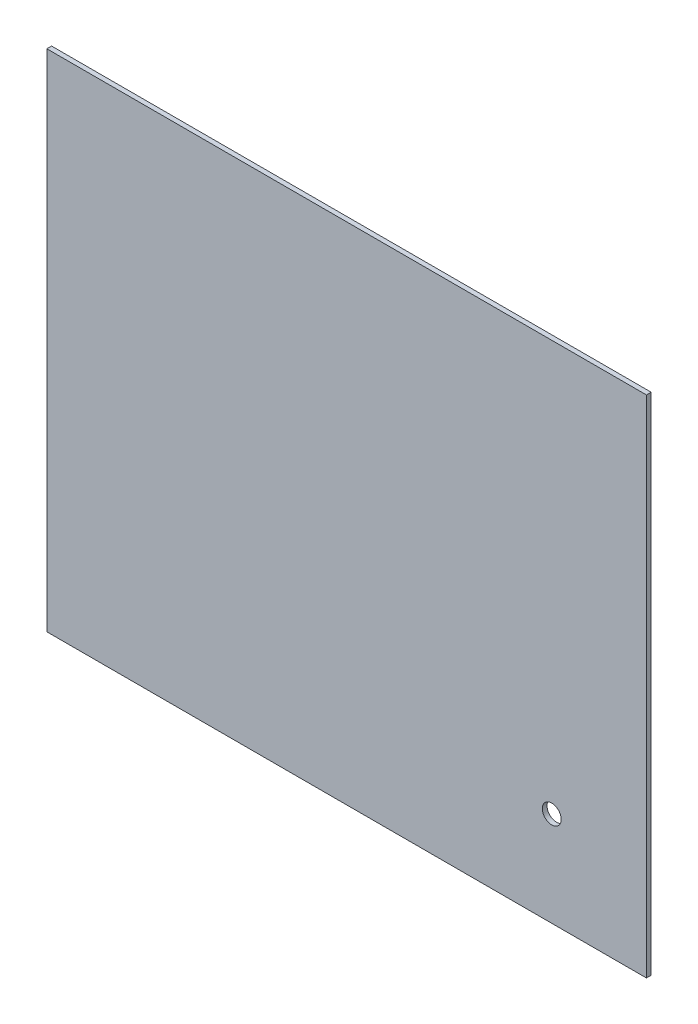
from build123d import *

# Parameters (mm, degrees)
SKETCH_1_W          = 380
SKETCH_1_H          = 320
EXTRUDE_1_DEPTH     = 1.5
SKETCH_2_R          = 6
CUT_EXTRUDE_1_DEPTH = 11.5


with BuildPart() as part:
    # 草图1 → 凸台-拉伸1 (new, symmetric)
    with BuildSketch(Plane.XY):
        Rectangle(SKETCH_1_W, SKETCH_1_H)
    extrude(amount=EXTRUDE_1_DEPTH, both=True)

    # 草图2 → 切除-拉伸1 (cut, symmetric)
    with BuildSketch(Plane.XY):
        with Locations((130, -100)):
            Circle(SKETCH_2_R)
    extrude(amount=CUT_EXTRUDE_1_DEPTH, both=True, mode=Mode.SUBTRACT)


solid = part.part
